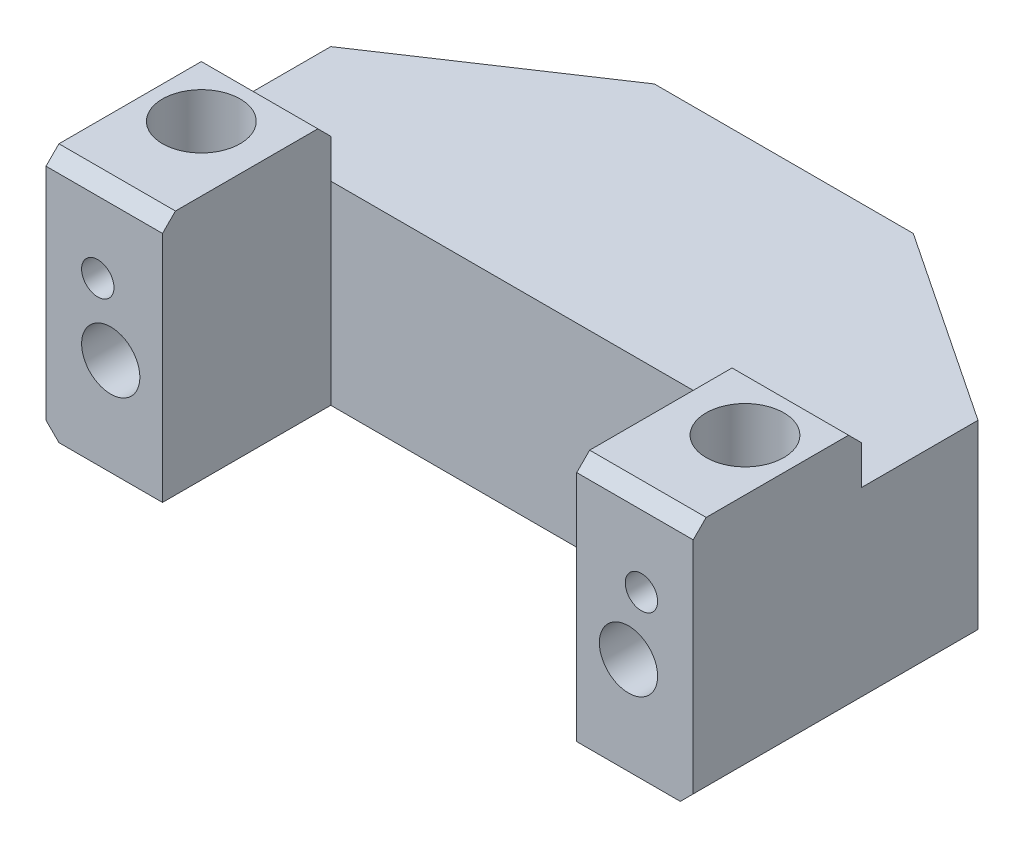
SolidWorks part; units mm, degrees
material "AISI 304"
ref_plane "Front Plane" through (0, 0, 0) normal (0, 0, 1) x (1, 0, 0)
ref_plane "Top Plane" through (0, 0, 0) normal (0, 1, 0) x (1, 0, 0)
ref_plane "Right Plane" through (0, 0, 0) normal (1, 0, 0) x (0, 0, -1)
sketch "Sketch1" plane through (0, 0, 0) normal (0, 1, 0) x (1, 0, 0)
  line L0 (0, 0) -> (0, -50000) construction
  line L1 (-25, 16) -> (25, 16)
  line L2 (-25, 16) -> (-25, -16)
  line L3 (-25, -16) -> (-16, -16)
  line L4 (25, 16) -> (25, -16)
  line L5 (-25, 16) -> (25, -16) construction
  line L6 (-25, -16) -> (25, 16) construction
  line L7 (16, -16) -> (25, -16)
  line L8 (-16, -3) -> (16, -3)
  line L9 (-16, -3) -> (-16, -16)
  line L11 (16, -3) -> (16, -16)
  line L12 (-16, -3) -> (16, -16) construction
  line L13 (-16, -16) -> (16, -3) construction
  point P0 (0, 0)
  point P8 (0, -9.5)
  dimension "D1" = 50
  dimension "D2" = 32
  dimension "D3" = 32
  dimension "D4" = 13
extrude "Boss-Extrude1" add sketch "Sketch1" along normal blind 15
chamfer "Chamfer1" distance 10 distance2 15 1 edges at (25, 7.5, -16)
chamfer "Chamfer2" distance 15 distance2 10 1 edges at (-25, 7.5, -16)
sketch "Sketch2" plane through (0, 0, -16) normal (0, 0, -1) x (-1, 0, 0)
  line L0 (0, 0) -> (0, 50000) construction
  line L1 (-10, 0) -> (-25, 0) construction
  circle A0 centre (-20, 7.5) radius 2.25
  circle A1 centre (20, 7.5) radius 2.25
  dimension "D1" = 40
  dimension "D2" = 4.5
  dimension "D3" = 7.5
extrude "Cut-Extrude1" cut sketch "Sketch2" against normal blind 36
sketch "Sketch3" plane through (0, 0, -16) normal (0, 0, -1) x (-1, 0, 0)
  circle A0 centre (-20, 7.5) radius 4
  circle A1 centre (20, 7.5) radius 4
  dimension "D1" = 8
extrude "Cut-Extrude2" cut sketch "Sketch3" against normal blind 13
sketch "Sketch12" plane through (0, 15, 0) normal (0, 1, 0) x (1, 0, 0)
  circle A0 centre (-21, -8) radius 3
  circle A1 centre (21, -8) radius 3
  dimension "D1" = 6
extrude "Cut-Extrude7" cut sketch "Sketch12" against normal blind 4.2
hole_wizard "M3 Tapped Hole1" positions "3DSketch1" profile "Sketch13" tap size "M3" standard "Gb"
sketch3d "3DSketch1"
  point P0 (-21, 12.5, 16)
  dimension "D1" = 4
  dimension "D2" = 2.5
sketch "Sketch13" plane through (-21, 12.5, 16) normal (1, 0, 0) x (0, -1, 0)
  line L0 (0, 0) -> (0, 8.2511)
  line L1 (0, 8.2511) -> (1.25, 7.5)
  line L2 (1.25, 7.5) -> (1.25, 0)
  line L5 (1.25, 0) -> (0, 0)
  line L10 (0, 8.2511) -> (-1.25, 7.5) construction
  line L11 (0, -6.35) -> (0, 107.95) construction
  dimension "螺纹孔钻头直径" = 2.5
  dimension "螺纹孔钻头深度" = 7.5
  dimension "导头角度" = 118
cosmetic thread "Hole thread1" parameters "D1"=5.2728, "D2"=3
hole_wizard "M3 Tapped Hole2" positions "3DSketch2" profile "Sketch14" tap size "M3" standard "Gb"
sketch3d "3DSketch2"
  point P0 (21, 12.5, 16)
  dimension "D1" = 4
  dimension "D2" = 2.5
sketch "Sketch14" plane through (21, 12.5, 16) normal (1, 0, 0) x (0, -1, 0)
  line L0 (0, 0) -> (0, 8.2511)
  line L1 (0, 8.2511) -> (1.25, 7.5)
  line L2 (1.25, 7.5) -> (1.25, 0)
  line L5 (1.25, 0) -> (0, 0)
  line L10 (0, 8.2511) -> (-1.25, 7.5) construction
  line L11 (0, -6.35) -> (0, 107.95) construction
  dimension "螺纹孔钻头直径" = 2.5
  dimension "螺纹孔钻头深度" = 7.5
  dimension "导头角度" = 118
cosmetic thread "Hole thread2" parameters "D1"=5.2728, "D2"=3
sketch "Sketch17" plane through (0, 15, 0) normal (0, 1, 0) x (1, 0, 0)
  line L1 (-16, -3) -> (-25, -3)
  line L2 (-16, -3) -> (-16, -16)
  line L3 (-16, -16) -> (-25, -16)
  line L4 (-25, -3) -> (-25, -16)
  line L5 (16, -3) -> (25, -3)
  line L6 (16, -3) -> (16, -16)
  line L7 (16, -16) -> (25, -16)
  line L8 (25, -3) -> (25, -16)
  circle A0 centre (21, -8) radius 3 construction
  circle A1 centre (-21, -8) radius 3 construction
  circle A2 centre (21, -8) radius 3
  circle A3 centre (-21, -8) radius 3
extrude "Boss-Extrude3" add sketch "Sketch17" along normal blind 4
sketch "Sketch18" plane through (0, 0, 0) normal (0, -1, 0) x (1, 0, 0)
  line L0 (10, -16) -> (-10, -16) construction
  line L1 (25, 16) -> (25, -6) construction
  circle A0 centre (0, -7.5) radius 5
  dimension "D2" = 25
  dimension "D3" = 10
  dimension "D1" = 8.5
extrude "Cut-Extrude8" cut sketch "Sketch18" against normal blind 8.2
chamfer "Chamfer3" distance 1 angle 45 6 edges at (-20.5, 19, 3) (20.5, 19, 3) (-20.5, 19, 16) (20.5, 19, 16) (-25, 0, 5) (25, 0, 5)
